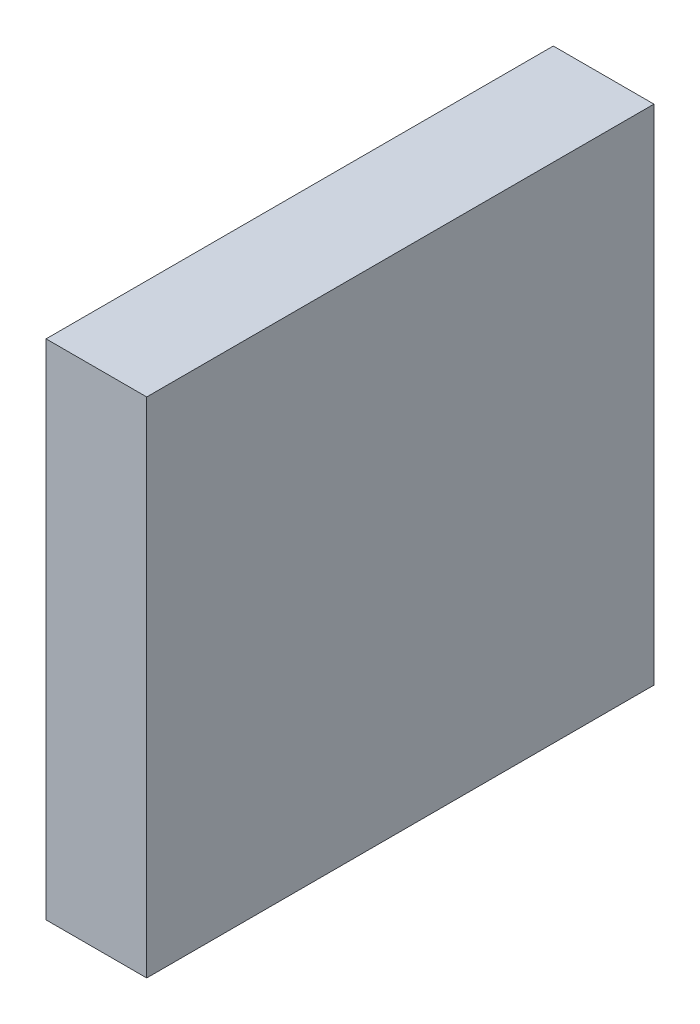
SolidWorks part; units mm, degrees
material "Q345B"
ref_plane "Front Plane" through (0, 0, 0) normal (0, 0, 1) x (1, 0, 0)
ref_plane "Top Plane" through (0, 0, 0) normal (0, 1, 0) x (1, 0, 0)
ref_plane "Right Plane" through (0, 0, 0) normal (1, 0, 0) x (0, 0, -1)
sketch "Sketch2" plane through (0, 0, 0) normal (0, 1, 0) x (1, 0, 0)
  line L0 (-131.395, 0) -> (113.7022, 0) construction
  line L1 (0, 164.1787) -> (0, -121.5078) construction
  line L3 (-12.5, 63) -> (12.5, 63)
  line L4 (-12.5, 63) -> (-12.5, -63)
  line L5 (-12.5, -63) -> (12.5, -63)
  line L6 (12.5, 63) -> (12.5, -63)
  dimension "D1" = 126
  dimension "D2" = 25
  dimension "D3" = 12.5
extrude "Boss-Extrude1" add sketch "Sketch2" along normal mid plane 125
